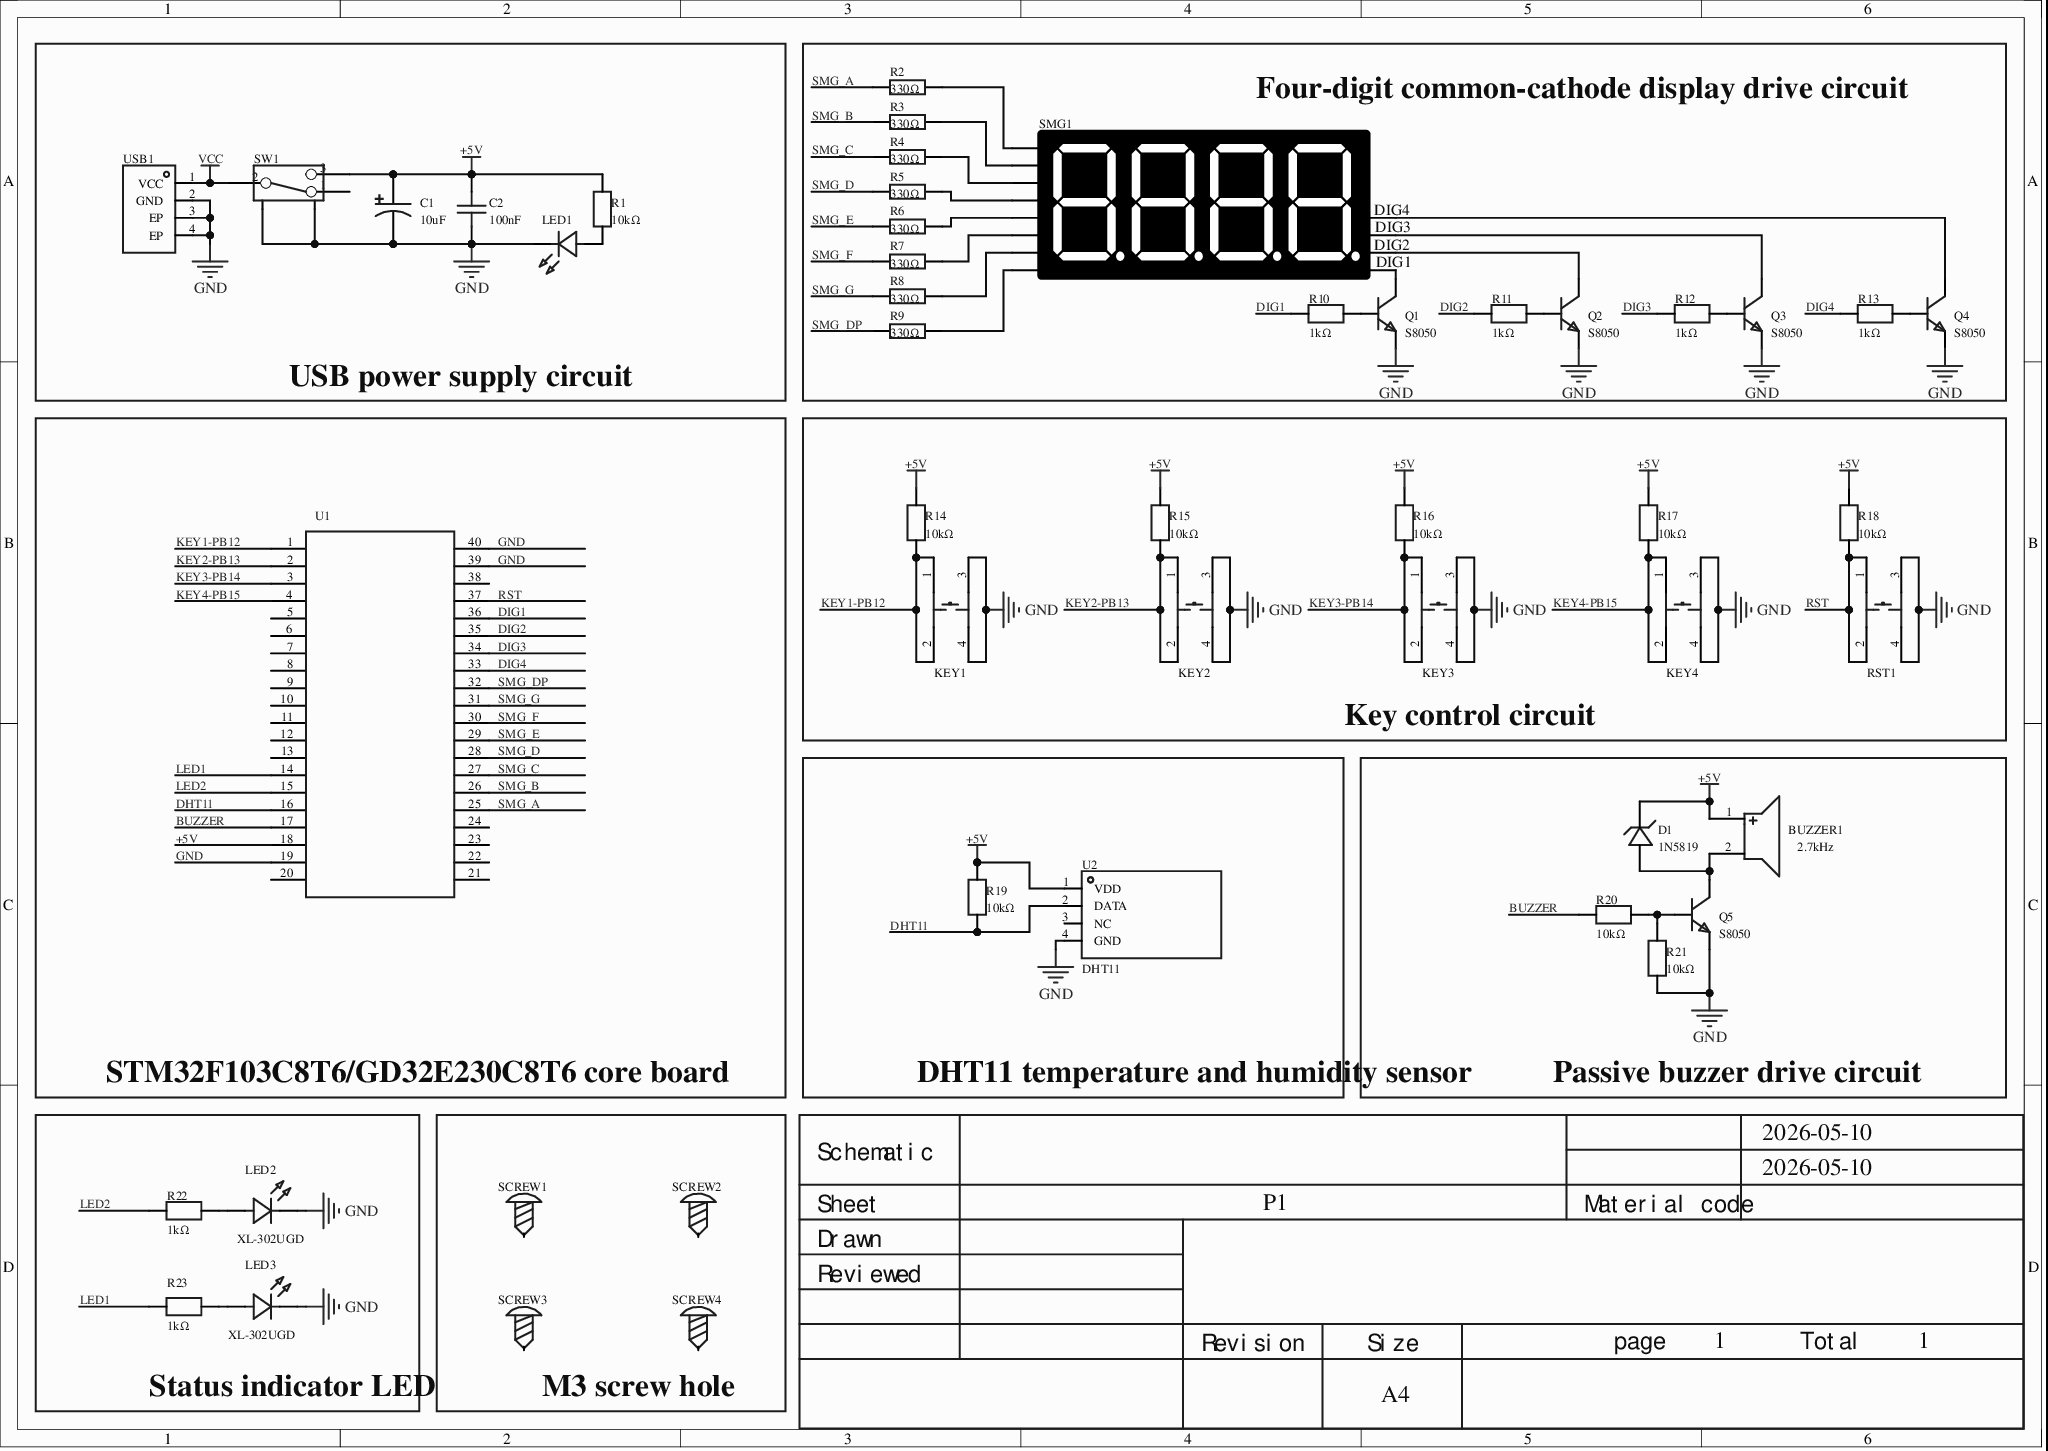
[diagram p0: MISC61551-3.schdoc]
# Altium project MISC61551-2.PrjPcb
1 sheet, 49 parts. Net scope: global (net labels, ports and power ports of the same name join across sheets).
Board file: MISC61551.pcbdoc

## Sheet MISC61551-3.schdoc
size 297 x 210 mm; Version: V1.0; @Project Name: MISC61551; @Page Count: 1; @Update Date: 2026-05-10; @Create Date: 2026-05-10; @Schematic Name: MISC61551; Part Number: MISC61551; @Page No: 1

### Parts
BUZZER1  2.7kHz  [BUZ-TH_BD9.0-P4.00-D0.6-FD]
C1  10uF  [CAP-TH_BD4.0-P1.50-D0.8-FD]
C2  100nF  [CAP-TH_L5.0-W2.5-P5.08-D0.7]
D1  1N5819  [DO-41_BD2.4-L4.7-P8.70-D0.9-RD]
KEY1  TS-1002-07026  [SW-TH_4P-L6.0-W6.0-P4.50-LS6.5]  (value not drawn)
KEY2  TS-1002-07026  [SW-TH_4P-L6.0-W6.0-P4.50-LS6.5]  (value not drawn)
KEY3  TS-1002-07026  [SW-TH_4P-L6.0-W6.0-P4.50-LS6.5]  (value not drawn)
KEY4  TS-1002-07026  [SW-TH_4P-L6.0-W6.0-P4.50-LS6.5]  (value not drawn)
LED1  XL-302SURD  [LED-TH_BD3.8-P2.54-RD]  (value not drawn)
LED2  XL-302UGD  [LED-TH_BD3.8-P2.54-FD_GREEN]
LED3  XL-302UGD  [LED-TH_BD3.8-P2.54-FD_GREEN]
Q1  S8050  [TO-92-3_L4.5-W3.5-P1.27-L]
Q2  S8050  [TO-92-3_L4.5-W3.5-P1.27-L]
Q3  S8050  [TO-92-3_L4.5-W3.5-P1.27-L]
Q4  S8050  [TO-92-3_L4.5-W3.5-P1.27-L]
Q5  S8050  [TO-92-3_L4.5-W3.5-P1.27-L]
R1  10kΩ  [RES-TH_BD2.4-L6.3-P10.30-D0.6]
R2  330Ω  [RES-TH_BD2.2-L6.5-P10.50-D0.6]
R3  330Ω  [RES-TH_BD2.2-L6.5-P10.50-D0.6]
R4  330Ω  [RES-TH_BD2.2-L6.5-P10.50-D0.6]
R5  330Ω  [RES-TH_BD2.2-L6.5-P10.50-D0.6]
R6  330Ω  [RES-TH_BD2.2-L6.5-P10.50-D0.6]
R7  330Ω  [RES-TH_BD2.2-L6.5-P10.50-D0.6]
R8  330Ω  [RES-TH_BD2.2-L6.5-P10.50-D0.6]
R9  330Ω  [RES-TH_BD2.2-L6.5-P10.50-D0.6]
R10  1kΩ  [RES-TH_BD2.2-L6.5-P10.50-D0.6]
R11  1kΩ  [RES-TH_BD2.2-L6.5-P10.50-D0.6]
R12  1kΩ  [RES-TH_BD2.2-L6.5-P10.50-D0.6]
R13  1kΩ  [RES-TH_BD2.2-L6.5-P10.50-D0.6]
R14  10kΩ  [RES-TH_BD2.4-L6.3-P10.30-D0.6]
R15  10kΩ  [RES-TH_BD2.4-L6.3-P10.30-D0.6]
R16  10kΩ  [RES-TH_BD2.4-L6.3-P10.30-D0.6]
R17  10kΩ  [RES-TH_BD2.4-L6.3-P10.30-D0.6]
R18  10kΩ  [RES-TH_BD2.4-L6.3-P10.30-D0.6]
R19  10kΩ  [RES-TH_BD2.4-L6.3-P10.30-D0.6]
R20  10kΩ  [RES-TH_BD2.4-L6.3-P10.30-D0.6]
R21  10kΩ  [RES-TH_BD2.4-L6.3-P10.30-D0.6]
R22  1kΩ  [RES-TH_BD2.2-L6.5-P10.50-D0.6]
R23  1kΩ  [RES-TH_BD2.2-L6.5-P10.50-D0.6]
RST1  TS-1002-07026  [SW-TH_4P-L6.0-W6.0-P4.50-LS6.5]  (value not drawn)
SCREW1  (no value)  [M3螺丝]
SCREW2  (no value)  [M3螺丝]
SCREW3  (no value)  [M3螺丝]
SCREW4  (no value)  [M3螺丝]
SMG1  (no value)  [LED-SEG-TH_FJ5461AH]
SW1  SK-12E12-G5  [SW-TH_SK-12E12-G5]  (value not drawn)
U1  GD32E230C8T6 minimum system board  [GD32E230C8T6最小系统]  (value not drawn)
U2  DHT11  [SENSOR-TH_DHT11]
USB1  KH-TYPE-C-2P  [USB-SMD_KH-TYPE-C-2P]  (value not drawn)

### Blocks framed on the sheet
USB power supply circuit: C1 C2 LED1 R1 SW1 USB1
Four-digit common-cathode display drive circuit: Q1-Q4 R2-R13 SMG1
STM32F103C8T6/GD32E230C8T6 core board: U1
Key control circuit: KEY1-KEY4 R14-R18 RST1
DHT11 temperature and humidity sensor: R19 U2
Passive buzzer drive circuit: BUZZER1 D1 Q5 R20 R21
Status indicator LED: LED2 LED3 R22 R23
M3 screw hole: SCREW1-SCREW4

### Nets
+5V: BUZZER1.1 C1.1 C2.2 D1.1(C) R1.2 R14.2 R15.2 R16.2 R17.2 R18.2 R19.2 SW1.3 U1.18(5V) U2.1(VDD)
GND: C1.2 C2.1 KEY1.3 KEY1.4 KEY2.3 KEY2.4 KEY3.3 KEY3.4 KEY4.3 KEY4.4 LED1.1(K) LED2.2(K) LED3.2(K) Q1.1(E) Q2.1(E) Q3.1(E) Q4.1(E) Q5.1(E) R21.1 RST1.3 RST1.4 SW1.4 SW1.5 U1.19(GND) U1.39(GND) U1.40(GND) U2.4(GND) USB1.2(GND) USB1.3(EP) USB1.4(EP)
VCC: SW1.2 USB1.1(VCC)
BUZZER: R20.2 U1.17(B09)
DHT11: R19.1 U1.16(B08) U2.2(DATA)
DIG1: R10.2 U1.36(B11)
DIG2: R11.2 U1.35(B10)
DIG3: R12.2 U1.34(B01)
DIG4: R13.2 U1.33(B00)
KEY1-PB12: KEY1.1 KEY1.2 R14.1 U1.1(B12)
KEY2-PB13: KEY2.1 KEY2.2 R15.1 U1.2(B13)
KEY3-PB14: KEY3.1 KEY3.2 R16.1 U1.3(B14)
KEY4-PB15: KEY4.1 KEY4.2 R17.1 U1.4(B15)
LED1: R23.2 U1.14(B06)
LED2: R22.2 U1.15(B07)
RST: R18.1 RST1.1 RST1.2 U1.37(RST)
SMG_A: R2.1 U1.25(A00)
SMG_B: R3.1 U1.26(A01)
SMG_C: R4.1 U1.27(A02)
SMG_D: R5.1 U1.28(A03)
SMG_DP: R9.1 U1.32(A07)
SMG_E: R6.1 U1.29(A04)
SMG_F: R7.1 U1.30(A05)
SMG_G: R8.1 U1.31(A06)
NetBUZZER1_2: BUZZER1.2 D1.2(A) Q5.3(C)
NetLED1_2: LED1.2(A) R1.1
NetLED2_1: LED2.1(A) R22.1
NetLED3_1: LED3.1(A) R23.1
NetQ1_2: Q1.2(B) R10.1
NetQ1_3: Q1.3(C) SMG1.12(DIG1)
NetQ2_2: Q2.2(B) R11.1
NetQ2_3: Q2.3(C) SMG1.9(DIG2)
NetQ3_2: Q3.2(B) R12.1
NetQ3_3: Q3.3(C) SMG1.8(DIG3)
NetQ4_2: Q4.2(B) R13.1
NetQ4_3: Q4.3(C) SMG1.6(DIG4)
NetQ5_2: Q5.2(B) R20.1 R21.2
NetR2_2: R2.2 SMG1.11(A)
NetR3_2: R3.2 SMG1.7(B)
NetR4_2: R4.2 SMG1.4(C)
NetR5_2: R5.2 SMG1.2(D)
NetR6_2: R6.2 SMG1.1(E)
NetR7_2: R7.2 SMG1.10(F)
NetR8_2: R8.2 SMG1.5(G)
NetR9_2: R9.2 SMG1.3(DP)

Not connected (* = marked no-connect by the designer): SCREW1 1*; SCREW2 1*; SCREW3 1*; SCREW4 1*; SW1 1*; U1 5(A08)* 6(A09)* 7(A10)* 8(A11)* 9(A12)* 10(A15)* 11(B03)* 12(B04)* 13(B05)* 20(3V3)* 21(BAT)* 22(C13)* 23(C14)* 24(C15)* 38(3V3)*; U2 3(NC)*

### Notes on the sheet
- 2026-05-10
- Schematic
- Sheet
- P1
- Material code
- Reviewed
- Drawn
- Revision
- Size
- A4
- page
- 1
- Total

### Library data of the parts
BUZZER1 = QMB-09B-03: Drive mode: passive (external drive); construction: electromagnetic; frequency: 2.7kHz; sound pressure (SPL): 85dB@3V,10cm;; Manufacturer: 华能; AddInBom: yes; ModelId: 949096c5110a440bbcfd89e7e6948986; ModelName: BUZ-TH_D9.0-H5.5-P4.0; ModelTransform: 354.33,354.33,0,90,0,0,0,0,-177.165; Operating Voltage: 2V~5V; Symbol: QMB-09B-03; Device: QMB-09B-03; Supplier: LCSC; Manufacturer Part: QMB-09B-03; Supplier Part: C96256; JLCPCB Part Class: Extended library; Value: 2.7kHz; LCSC Part Name: 无源蜂鸣器QMB-09B-03; Supplier Footprint: 插件,D=9mm; Datasheet: https://atta.szlcsc.com/upload/public/pdf/source/20210401/C96256_958B17753B5AD7CBFBCFFC7C095B4484.pdf; ConvertToPcb: yes; FootprintName: BUZ-TH_BD9.0-P4.00-D0.6-FD; Oscillator Circuit: Passive (external drive); Technology Type: Electromagnetic; Sound Pressure Level (SPL): 85dB@3V,10cm; Diameter (φD): 9mm; Height: 5.7mm
C1 = KF1E100MB050A00CV0: Capacitance: 10uF; tolerance: ±20%; rated voltage: 25V;; Manufacturer: HUAWEI(华威集团); AddInBom: yes; ModelId: 8017ea3dd4884afab5fc61dd7898abc1; ModelName: CAP-TH_D4.0-H7.0-P1.5; ModelTransform: 158.2674,157.45008,0,0,0,0,0,0,-137.795; φD: 4mm; L: 5mm; Lifetime @ Temp: 1000hrs@105℃; Device: KF1E100MB050A00CV0; Symbol: KF1E100MB050A00CV0; LCSC Part Name: 10uF ±20% 25V; SupplierPart: C216306; ManufacturerPart: KF1E100MB050A00CV0; Supplier Footprint: 插件,D4xL5mm; JLCPCB Part Class: Extended library; Datasheet: https://atta.szlcsc.com/upload/public/pdf/source/20181022/C271305_EAB36A8975ADE9B953FB348CB9D3587F.pdf; Supplier: LCSC; ConvertToPcb: yes; FootprintName: CAP-TH_BD4.0-P1.50-D0.8-FD; Value: 10uF; Tolerance: ±20%; Rated Voltage: 25V; Lead Spacing: 1.5mm
C2 = CC1H104ZC74D3F5O30MN: Capacitance: 100nF; tolerance: -20%~+80%; rated voltage: 50V; temperature coefficient: Y5V;; Manufacturer: Dersonic(德尔创); AddInBom: yes; ModelId: 3d005bb2736f4b028b929daf59d2a504; ModelName: CAP-TH_L5.0-W2.5-P5.08; ModelTransform: 222.8342,98.419,0,0,0,0,0,0,-118.11; φD: 5.3mm; Body Thickness: 2.2mm; Symbol: CC1H104ZC74D3F5O30MN; Device: CC1H104ZC74D3F5O30MN; Supplier: LCSC; Supplier Part: C254094; Manufacturer Part: CC1H104ZC74D3F5O30MN; Value: 100nF; JLCPCB Part Class: Extended library; LCSC Part Name: 100nF -20%~+80% 50V; Supplier Footprint: 插件,P=5.08mm; Datasheet: https://atta.szlcsc.com/upload/public/pdf/source/20200826/C254094_5CB2628DB82B55380EF0EA1FCCF0C073.pdf; ConvertToPcb: yes; FootprintName: CAP-TH_L5.0-W2.5-P5.08-D0.7; Tolerance: -20%~+80%; Voltage Rated: 50V; Lead Spacing: 5.08mm; Temperature Coefficient: Y5V
D1 = 1N5819_C402218: Forward voltage drop (Vf): 900mV@3A; DC reverse withstand voltage (Vr): 40V; average rectified current (Io): 1A;; Manufacturer: LGE(鲁光); AddInBom: yes; ModelId: 6de1e9b71a0d4751b4e9df530304c1a3; ModelName: DO-41_D2.4-L4.7-P8.70; ModelTransform: 374.016,94.488,0,0,0,0,0,0,-137.795; Symbol: 1N5819_C402218; Device: 1N5819_C402218; Supplier: LCSC; Supplier Part: C402218; Manufacturer Part: 1N5819; JLCPCB Part Class: Extended library; LCSC Part Name: 电压:40V 电流:1A; Supplier Footprint: DO-41; Datasheet: https://atta.szlcsc.com/upload/public/pdf/source/20190705/C402218_ECB4BB85D6DB51BBD80C05504B9336F4.pdf; ConvertToPcb: yes; FootprintName: DO-41_BD2.4-L4.7-P8.70-D0.9-RD; Forward Voltage (Vf@If): 900mV@3A; Reverse Voltage (Vr): 40V; Average Rectified Current (Io): 1A
KEY1-KEY4 RST1 = TS-1002-07026: Circuit structure: single pole single throw; button shape: round button; mounting: through-hole; switch length: 6mm; switch width: 6mm; switch height: 7mm; contact current: 50mA; rated voltage (DC): 12V; with light: -; mechanical life: -;; Manufacturer: XUNPU(讯普); AddInBom: yes; ModelId: 20eee248bc684ccd8cbdbb1d0d91ec6f; ModelName: SW-TH_4P-L6.0-W6.0-H5.0-LS6.5-P4.50; ModelTransform: 236.22,323.03,0,90,0,0,0,0,-137.795; Symbol: TS-1002-07026; Device: TS-1002-07026; Supplier: LCSC; Supplier Part: C455095; Manufacturer Part: TS-1002-07026; JLCPCB Part Class: Extended library; LCSC Part Name: 6*6*7mm 直插 轻触开关; Supplier Footprint: 插件,6x6mm; Datasheet: https://atta.szlcsc.com/upload/public/pdf/source/20231108/52BC6409AB52B6746CCC051A15664904.pdf; ConvertToPcb: yes; FootprintName: SW-TH_4P-L6.0-W6.0-P4.50-LS6.5; Circuit: Single pole single throw; Actuator Style: Round button; Mounting Style: Through-hole; Switch Length: 6mm; Switch Width: 6mm; Switch Height: 7mm; Contact Current: 50mA; Voltage Rating (DC): 12V; With Lamp: -; Mechanical Life: -
LED1 = XL-302SURD: Lamp head type: 3mm round lamp head; emitted color: red; power: 80mW; forward current: 30mA; dominant wavelength: 615nm~620nm; lens color: red lens; color temperature: -; viewing angle: 50°; tape and reel: -; operating temperature: -25℃~+85℃;; Manufacturer: XINGLIGHT(成兴光); AddInBom: yes; ModelId: 6a9b7f7cc45d49ea908a5f911cd0be96; ModelTransform: 134.372,149.6,0,180,0,0,6.89,0,-196.85; Peak Wavelength: 625nm; Symbol: XL-302SURD; Device: XL-302SURD; LCSC Part Name: XL-302SURD; SupplierPart: C2895470; ManufacturerPart: XL-302SURD; Supplier Footprint: 插件,D=3mm; JLCPCB Part Class: Extended library; Datasheet: https://atta.szlcsc.com/upload/public/pdf/source/20240112/E1E2B82945FD635E4907401DDE6D4922.pdf; Supplier: LCSC; ConvertToPcb: yes; FootprintName: LED-TH_BD3.8-P2.54-RD; ModelName: LED-TH_BD3.8-P2.54-RD; Lamp Holder Type: 3mm round lamp head; Emitted Color: Red; Power Dissipation: 80mW; Forward Current: 30mA; Dominant Wavelength: 615nm~620nm; Lens Color: Red lens; Color Temperature: -; Viewing Angle: 50°; Mounting Sytle: -; Operating Temperature: -25℃~+85℃
LED2 LED3 = XL-302UGD: Lamp head type: 3mm round lamp head; emitted color: emerald green; power: 80mW; forward current: 30mA; dominant wavelength: 510nm~520nm; lens color: green lens; color temperature: -; viewing angle: 50°; tape and reel: -; operating temperature: -25℃~+85℃;; Manufacturer: XINGLIGHT(成兴光); AddInBom: yes; ModelId: c917953ee2724e1d8eea37a428b0e119; ModelTransform: 134.40603,149.41647,0,0,0,0,-7.874,0,-137.795; Peak Wavelength: 525nm; Symbol: XL-302UGD; Device: XL-302UGD; LCSC Part Name: XL-302UGD; SupplierPart: C2895476; ManufacturerPart: XL-302UGD; Supplier Footprint: 插件,D=3mm; JLCPCB Part Class: Extended library; Datasheet: https://atta.szlcsc.com/upload/public/pdf/source/20240112/A4C1FE2F91E20BD07CDB872CEF78D7A0.pdf; Supplier: LCSC; ConvertToPcb: yes; FootprintName: LED-TH_BD3.8-P2.54-FD_GREEN; ModelName: LED-TH_BD3.8-P2.54-FD_GREEN; Lamp Holder Type: 3mm round lamp head; Emitted Color: Emerald green; Power Dissipation: 80mW; Forward Current: 30mA; Dominant Wavelength: 510nm~520nm; Lens Color: Green lens; Color Temperature: -; Viewing Angle: 50°; Mounting Sytle: -; Operating Temperature: -25℃~+85℃
Q1-Q5 = S8050_C2931492: Transistor type: NPN; collector current (Ic): 500mA; collector-emitter breakdown voltage (Vceo): 25V; power (Pd): 625mW; DC current gain (hFE@Ic,Vce): 160@50mA,1V;; Manufacturer: JSMSEMI(杰盛微); AddInBom: yes; ModelId: 45fa6cddef3743c6aacf8db740a3bc4c; ModelTransform: 177.165,137.795,0,0,0,0,0,29.528,-98.425; Transition Frequency (fT): 150MHz; Collector Cut-Off Current (Icbo): 100nA; Collector-Emitter Saturation Voltage (VCE(sat)@Ic,Ib): 600mV@500mA,50mA; Symbol: S8050_C2931492; Device: S8050_C2931492; LCSC Part Name: NPN 电流:500mA 耐压:25V; SupplierPart: C2931492; ManufacturerPart: S8050; Supplier Footprint: TO-92-3; JLCPCB Part Class: Extended library; Datasheet: https://atta.szlcsc.com/upload/public/pdf/source/20240105/D4E57AD221AC7DEA1E31B953388D993E.pdf; Supplier: LCSC; ConvertToPcb: yes; FootprintName: TO-92-3_L4.5-W3.5-P1.27-L; ModelName: TO-92-3_L4.5-W3.5-P1.27-L; Transistor Type: NPN; Collector Current (Ic): 500mA; Collector-Emitter Breakdown Voltage (Vceo): 25V; Power Dissipation (Pd): 625mW; DC Current Gain (hFE@Ic,Vce): 160@50mA,1V
R1 R14-R21 = MFR-25JT-52-10K: Resistor type: metal film resistor; resistance: 10kΩ; tolerance: ±5%; power: 250mW;; Manufacturer: YAGEO(国巨); Overload Voltage (Max): 250V; Temperature Coefficient: ±100ppm/℃; Symbol: MF1/4W-10K±1%-ST52; AddInBom: yes; ModelId: 463263665006444ab7a47bd11b0cf956; ModelTransform: 427.165,94.32816,0,0,0,0,0,0,-196.85; Device: MFR-25JT-52-10K; LCSC Part Name: 金属膜电阻 10kΩ ±5% 250mW; SupplierPart: C176451; ManufacturerPart: MFR-25JT-52-10K; Supplier Footprint: 插件; JLCPCB Part Class: Extended Part; Datasheet: https://atta.szlcsc.com/upload/public/pdf/source/20191118/C457825_18355E864DE4965678DC27B0EBC3E21E.pdf; Supplier: LCSC; ConvertToPcb: yes; FootprintName: RES-TH_BD2.4-L6.3-P10.30-D0.6; ModelName: RES-TH_BD2.4-L6.3-P10.30-D0.6; Type: Metal film resistor; Value: 10kΩ; Tolerance: ±5%; Power(Watts): 250mW; Operating Temperature Range: -55℃~+155℃
R2-R9 = MFR-25FTE52-330R: Resistor type: metal film resistor; resistance: 330Ω; tolerance: ±1%; power: 250mW; temperature coefficient: ±50ppm/℃;; Manufacturer: YAGEO(国巨); Symbol: MFR0W4F3300A50; Overload Voltage (Max): 250V; AddInBom: yes; ModelId: b909c601053f4d6186ab8392cbab0ca9; ModelName: RES-TH_BD2.2-L6.5-P10.50; ModelTransform: 431.1015,91.3384,0,0,0,0,-0.002,0,-137.795; Device: MFR-25FTE52-330R; Supplier: LCSC; Manufacturer Part: MFR-25FTE52-330R; Supplier Part: C138208; Value: 330Ω; JLCPCB Part Class: Extended Part; LCSC Part Name: 金属膜电阻 330Ω ±1% 250mW; Supplier Footprint: 插件,D2.4xL6.3mm; Datasheet: https://atta.szlcsc.com/upload/public/pdf/source/20191118/C457825_18355E864DE4965678DC27B0EBC3E21E.pdf; ConvertToPcb: yes; FootprintName: RES-TH_BD2.2-L6.5-P10.50-D0.6; Type: Metal film resistor; Tolerance: ±1%; Power(Watts): 250mW; Temperature Coefficient: ±50ppm/℃; Operating Temperature Range: -55℃~+155℃
R10-R13 R22 R23 = MFR-25JT-52-1K: Resistor type: metal film resistor; resistance: 1kΩ; tolerance: ±5%; power: 250mW;; Manufacturer: YAGEO(国巨); Temperature Coefficient: ±200ppm/℃; Symbol: MF1/4W-1KΩ±1%T52; AddInBom: yes; ModelId: b909c601053f4d6186ab8392cbab0ca9; ModelName: RES-TH_BD2.2-L6.5-P10.50; ModelTransform: 431.1015,91.3384,0,0,0,0,-0.002,0,-137.795; Device: MFR-25JT-52-1K; LCSC Part Name: 金属膜电阻 1kΩ ±5% 250mW; SupplierPart: C176465; ManufacturerPart: MFR-25JT-52-1K; Supplier Footprint: 插件; JLCPCB Part Class: Extended Part; Datasheet: https://atta.szlcsc.com/upload/public/pdf/source/20191118/C457825_18355E864DE4965678DC27B0EBC3E21E.pdf; Supplier: LCSC; ConvertToPcb: yes; FootprintName: RES-TH_BD2.2-L6.5-P10.50-D0.6; Type: Metal film resistor; Value: 1kΩ; Tolerance: ±5%; Power(Watts): 250mW; Operating Temperature Range: -55℃~+155℃
SCREW1-SCREW4 = M3螺丝: Device: M3 screw; ConvertToPcb: yes; SymbolName: Screw hole; AddInBom: yes; Supplier Footprint: 插件; FootprintName: M3 screw
SMG1 = LED_SEG_TH_0.56x4: ConvertToPcb: yes; ModelId: 40bbdb961cbb4a37879849f9a42b8331; ModelName: LED-SEG-TH_12P-L50.2-W19.0-H8.0-P2.54-S15.24; ModelTransform: 1976.37408,748.03,0,0,0,0,0,0,-137.795; Device: LED_SEG_TH_0.56x4; Symbol: LED_SEG_TH_0.56x4; AddInBom: yes; Supplier Footprint: 插件; FootprintName: LED-SEG-TH_FJ5461AH
SW1 = SK-12E12-G5: Circuit structure: single pole double throw; mounting: side entry; rated current (DC): -; rated voltage (DC): -; rated current (AC): -; rated voltage (AC): -; mechanical life: 5 thousand cycles;; Manufacturer: 韩国韩荣; AddInBom: yes; ModelId: 63ecb7c3b60e41c79481f203e3e77e6b; ModelTransform: 507.874,401.575,0,90,0,0,105,0,-137.795; Actuator Style: Rectangular post; Pin Style: PC pin; Switch Height: 10.6mm; Symbol: SK-12E12-G5; Device: SK-12E12-G5; LCSC Part Name: 卧插双档 滑动开关; SupplierPart: C136720; ManufacturerPart: SK-12E12-G5; Supplier Footprint: 插件; JLCPCB Part Class: Extended library; Datasheet: https://atta.szlcsc.com/upload/public/pdf/source/20210810/880D64C2F8CCE477762EFCC00B7B7681.pdf; Supplier: LCSC; ConvertToPcb: yes; FootprintName: SW-TH_SK-12E12-G5; ModelName: SW-TH_SK-12E12-G5; Circuit: Single pole double throw; Mounting Style: Side entry; Current Rating (DC): -; Voltage Rating (DC): -; Current Rating (AC): -; Voltage Rating (AC): -; Mechanical Life: 5 thousand cycles; Operating Temperature: -25℃~+70℃
U1 = GD32E230C8T6最小系统板: Manufacturer Part: C20068939; Manufacturer: 立创商城; AddInBom: yes; ModelId: f9b8c9e595d94a808d0aa286210d0cfc; ModelTransform: 2316.14,899,710.24,270,0,0,302.46,-1040.55,0; Device: GD32E230C8T6 minimum system board; ConvertToPcb: yes; SymbolName: GD32E230C8T6 minimum system board; FootprintName: GD32E230C8T6 minimum system; ModelName: GD32E230C8T6 minimum system board
U2 = DHT11: New capacitive digital temperature and humidity sensor; old version discontinued; 16.1x12.6x5.8mm; Manufacturer: 广州奥松; AddInBom: yes; ModelId: 6dde47d4d8bf4fa598dffcc067449c1d; ModelTransform: 236.25937,492.125,0,270,0,0,0,-11.811,-196.85; Symbol: DHT11; Device: DHT11; Supplier: LCSC; Supplier Part: C117051; Manufacturer Part: DHT11; JLCPCB Part Class: Extended library; LCSC Part Name: DHT11  电容式传感器; Supplier Footprint: SIP-4; Datasheet: https://atta.szlcsc.com/upload/public/pdf/source/20170703/1499081238365.pdf; ConvertToPcb: yes; FootprintName: SENSOR-TH_DHT11; ModelName: SENSOR-TH_DHT11
USB1 = KH-TYPE-C-2P: Connector type: -; standard: -; male/female: -; number of contacts: -; number of ports: -; mounting: -; rated current - power: -; contact material: -; contact plating: -; operating temperature range: -;; Manufacturer: kinghelm(金航标); AddInBom: yes; ModelId: 4464b34a7d0f48c2b8c2350e914c93f5; ModelTransform: 352.362,255.31449,0,0,0,0,0,-49.213,-98.425; Symbol: KH-TYPE-C-2P; Device: KH-TYPE-C-2P; Supplier: LCSC; Supplier Part: C2919656; Manufacturer Part: KH-TYPE-C-2P; JLCPCB Part Class: Extended library; LCSC Part Name: KH-TYPE-C-2P; Supplier Footprint: 插件; Datasheet: https://atta.szlcsc.com/upload/public/pdf/source/20220707/620587A9E0589B27D96D3CEE595CBC98.pdf; ConvertToPcb: yes; FootprintName: USB-SMD_KH-TYPE-C-2P; ModelName: USB-SMD_KH-TYPE-C-2P; Connector Type: -; Standard: -; Gender: -; Number of Contacts: -; Number of Ports: -; Mounting Style: -; Current Rating - Power (Max): -; Contact Material: -; Contact Plating: -; Operating Temperature Range: -